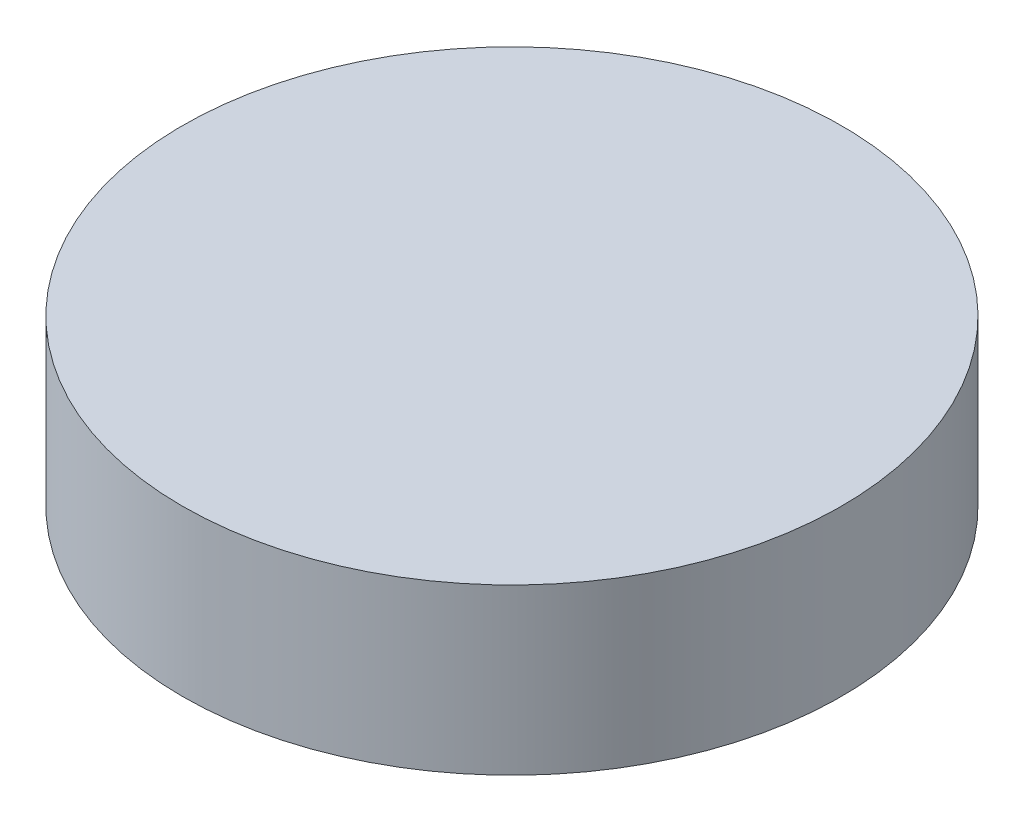
SolidWorks part; units mm, degrees
ref_plane "Front Plane" through (0, 0, 0) normal (0, 0, 1) x (1, 0, 0)
ref_plane "Top Plane" through (0, 0, 0) normal (0, 1, 0) x (1, 0, 0)
ref_plane "Right Plane" through (0, 0, 0) normal (1, 0, 0) x (0, 0, -1)
sketch "Sketch1" plane through (0, 0, 0) normal (0, 1, 0) x (1, 0, 0)
  circle A0 centre (0, 0) radius 4
  dimension "D1" = 8
extrude "Boss-Extrude1" add sketch "Sketch1" along normal blind 2
